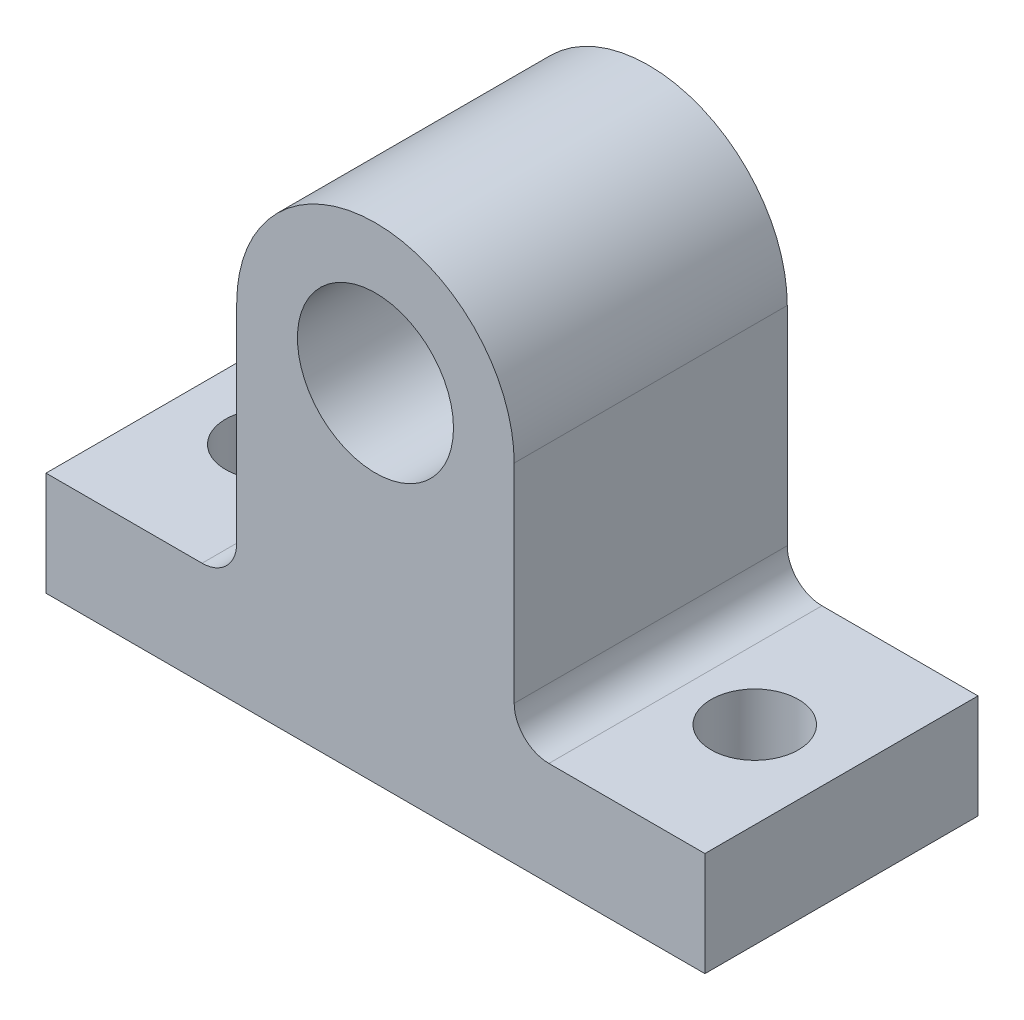
from build123d import *

# Parameters (mm, degrees)
SKETCH1_R          = 14.2875
EXTRUDE1_DEPTH     = 25
FILLET1_R          = 6.35
SKETCH2_R          = 8.001
CUT_EXTRUDE1_DEPTH = 92.084332489


with BuildPart() as part:
    # Sketch1 → Extrude1 (new, symmetric)
    with BuildSketch(Plane.XY):
        with BuildLine():
            Line((-25.4, 0), (-25.4, -44.45))
            Line((-25.4, -44.45), (-60.325, -44.45))
            Line((-60.325, -44.45), (-60.325, -63.5))
            Line((-60.325, -63.5), (60.325, -63.5))
            Line((60.325, -63.5), (60.325, -44.45))
            Line((60.325, -44.45), (25.4, -44.45))
            Line((25.4, -44.45), (25.4, 0))
            ThreePointArc((25.4, 0), (0, 25.4), (-25.4, 0))
        make_face()
        Circle(SKETCH1_R, mode=Mode.SUBTRACT)
    extrude(amount=EXTRUDE1_DEPTH, both=True)

    # Fillet1
    fillet1_edges = [part.edges().sort_by_distance(p)[0] for p in [
        (25.4, -44.45, 0),
        (-25.4, -44.45, 0),
    ]]
    fillet(fillet1_edges, radius=FILLET1_R)

    # Sketch2 → Cut-Extrude1 (cut, through all)
    with BuildSketch(Plane(origin=(0, 0, 0), x_dir=(1, 0, 0), z_dir=(0, 1, 0))):
        with Locations(Location((44.45, 0, 0), (0, 0, 270))):
            Circle(SKETCH2_R)
        with Locations(Location((-44.45, 0, 0), (0, 0, 90))):
            Circle(SKETCH2_R)
    extrude(amount=-CUT_EXTRUDE1_DEPTH, mode=Mode.SUBTRACT)


solid = part.part
